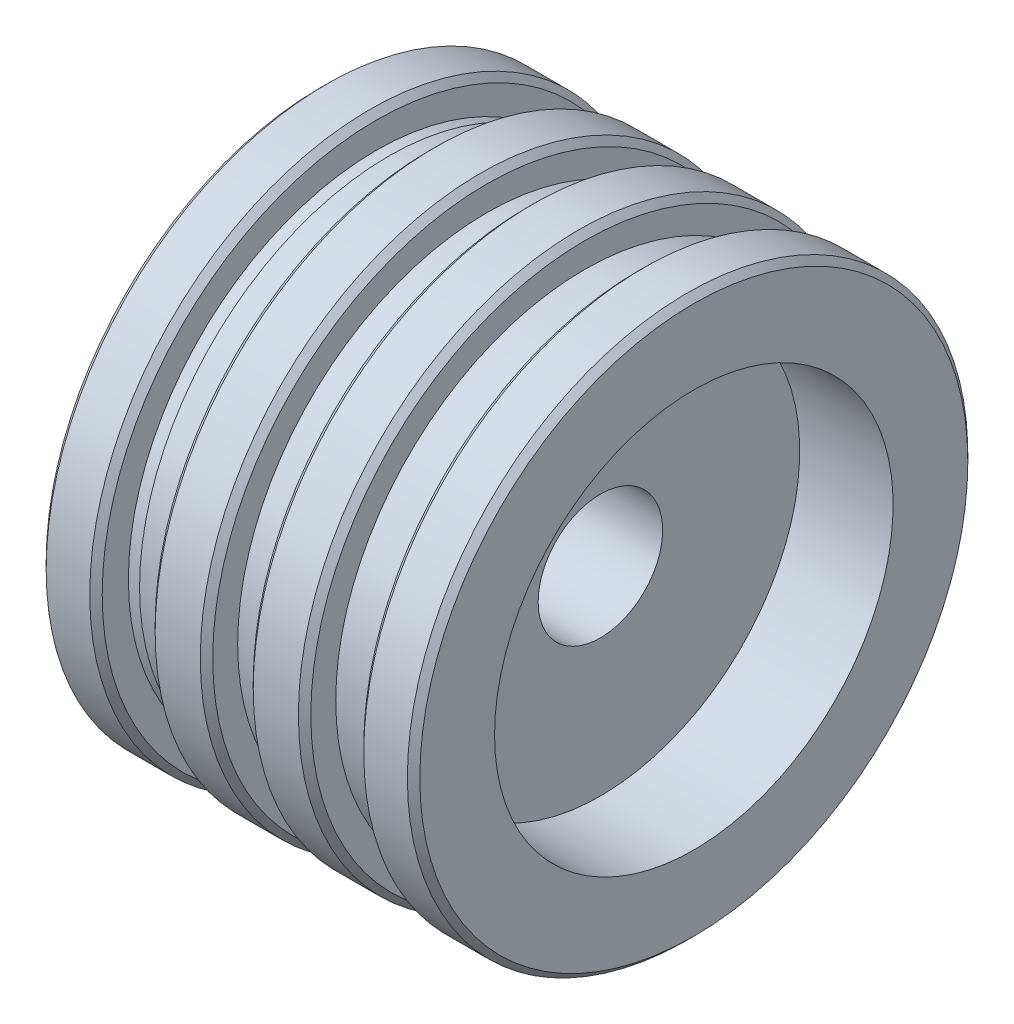
from build123d import *

# Parameters (mm, degrees)
CHAMFER_1_SIZE = 1


with BuildPart() as part:
    # 草图1 → 旋转1 (revolve)
    with BuildSketch(Plane(origin=(0, 0, 0), x_dir=(1, 0, 0), z_dir=(0, 1, 0)), mode=Mode.PRIVATE) as revolve_1_sk:
        Polygon((0, 16), (0, 45), (9, 45), (9, 39.8), (11, 39.8), (11, 40), (17.5, 40), (17.5, 45), (26.75, 45), (26.75, 40), (33.25, 40), (33.25, 45), (42.5, 45), (42.5, 40), (49, 40), (49, 39.8), (51, 39.8), (51, 45), (60, 45), (60, 32), (45, 32), (45, 10), (30, 10), (30, 16), align=None)
    revolve(revolve_1_sk.sketch.rotate(Axis((0, 0, 0), (1, 0, 0)), 180), axis=Axis((0, 0, 0), (1, 0, 0)))

    # 倒角1
    chamfer_1_edges = [part.edges().sort_by_distance(p)[0] for p in [
        (60, 0, -45),
        (51, 0, -45),
        (42.5, 0, -45),
        (33.25, 0, -45),
        (26.75, 0, -45),
        (17.5, 0, -45),
        (9, 0, -45),
        (0, 0, -45),
    ]]
    chamfer(chamfer_1_edges, length=CHAMFER_1_SIZE)


solid = part.part
